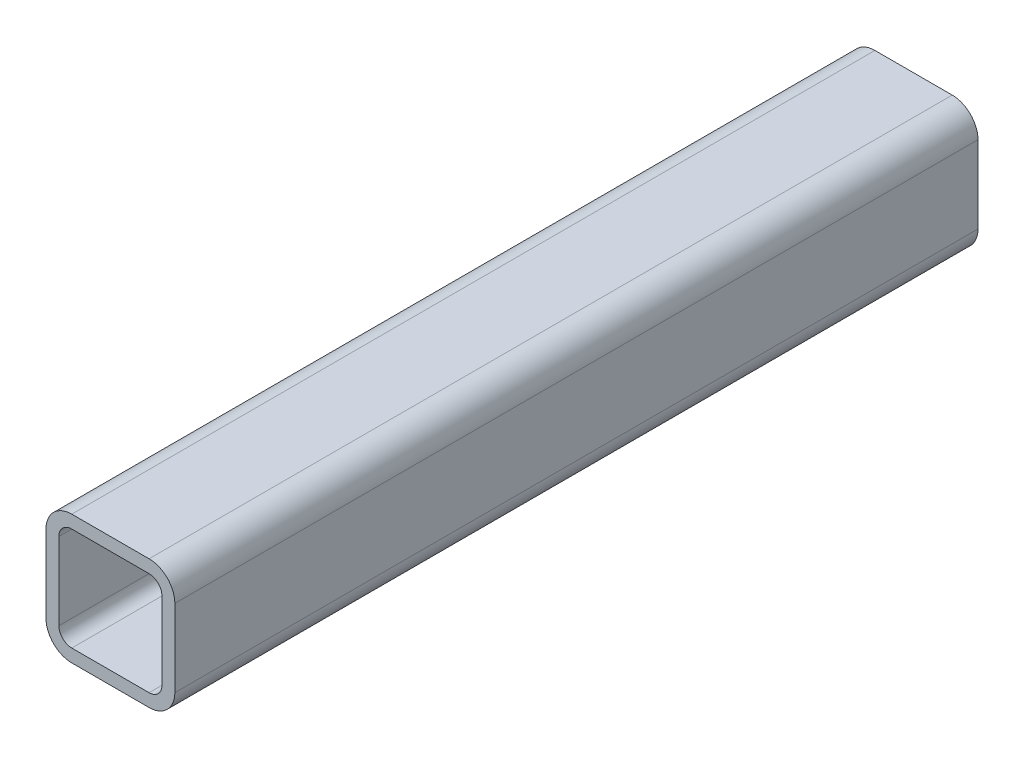
from build123d import *

# Parameters (mm, degrees)
BOSS_EXTRUDE1_DEPTH = 187


with BuildPart() as part:
    # Sketch1 → Boss-Extrude1 (new body)
    with BuildSketch(Plane.XY):
        with BuildLine():
            Line((-9, -15), (9, -15))
            ThreePointArc((9, -15), (13.242640687, -13.242640687), (15, -9))
            Line((15, -9), (15, 9))
            ThreePointArc((15, 9), (13.242640687, 13.242640687), (9, 15))
            Line((9, 15), (-9, 15))
            ThreePointArc((-9, 15), (-13.242640687, 13.242640687), (-15, 9))
            Line((-15, 9), (-15, -9))
            ThreePointArc((-15, -9), (-13.242640687, -13.242640687), (-9, -15))
        make_face()
        with BuildLine():
            Line((-9, -12), (9, -12))
            ThreePointArc((9, -12), (11.121320344, -11.121320344), (12, -9))
            Line((12, -9), (12, 9))
            ThreePointArc((12, 9), (11.121320344, 11.121320344), (9, 12))
            Line((9, 12), (-9, 12))
            ThreePointArc((-9, 12), (-11.121320344, 11.121320344), (-12, 9))
            Line((-12, 9), (-12, -9))
            ThreePointArc((-12, -9), (-11.121320344, -11.121320344), (-9, -12))
        make_face(mode=Mode.SUBTRACT)
    extrude(amount=BOSS_EXTRUDE1_DEPTH)


solid = part.part
